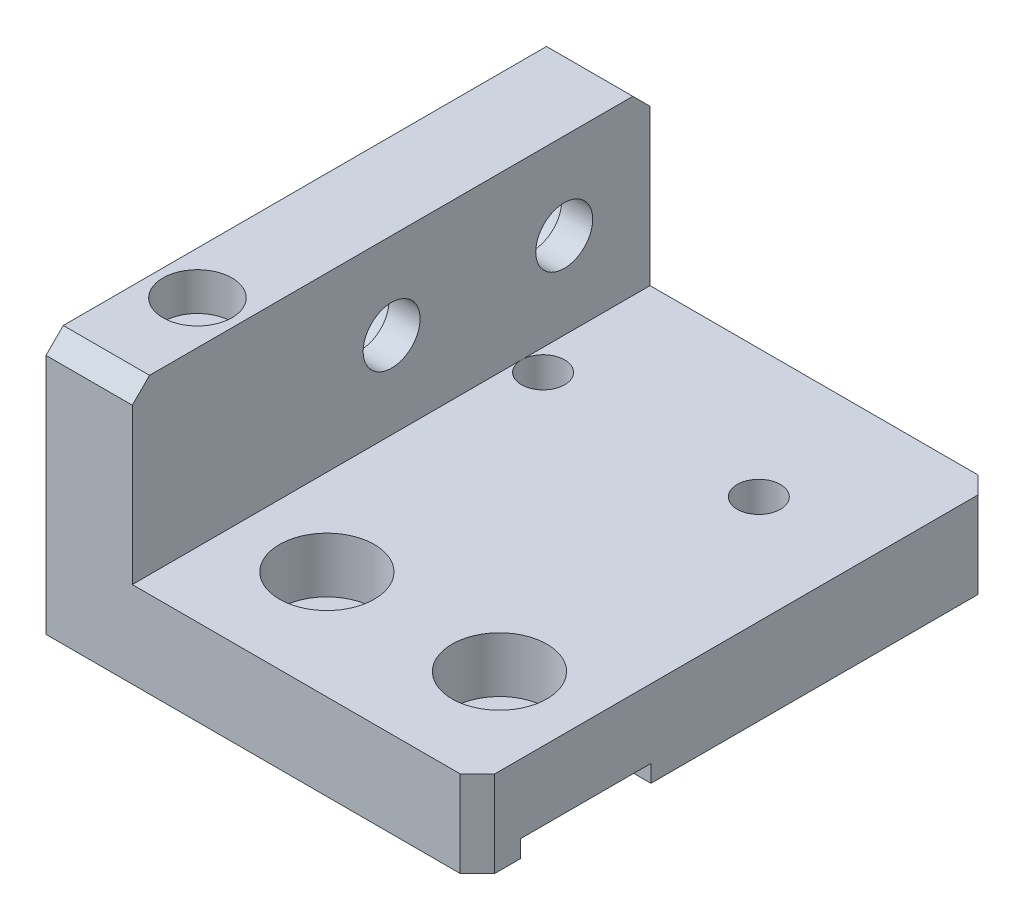
from build123d import *

# Parameters (mm, degrees)
EXTRUDE_1_DEPTH              = 60
SKETCH_3_W                   = 50
SKETCH_3_H                   = 15.1
CUT_EXTRUDE_1_DEPTH          = 2
HOLE_WIZARD_M4_1_D           = 4.5
HOLE_WIZARD_M4_1_CBORE_D     = 8
HOLE_WIZARD_M4_1_CBORE_DEPTH = 4.4
HOLE_WIZARD_M6_1_D           = 6.6
HOLE_WIZARD_M6_1_CBORE_D     = 11
HOLE_WIZARD_M6_1_CBORE_DEPTH = 6.4
HOLE_WIZARD_M6_2_D           = 6.6
HOLE_WIZARD_M6_2_CBORE_D     = 11
HOLE_WIZARD_M6_2_CBORE_DEPTH = 6.4
CHAMFER_1_SIZE               = 2
HOLE_WIZARD_M6_1_2_D         = 5
HOLE_WIZARD_M6_1_2_DEPTH     = 17
HOLE_WIZARD_M6_1_2_TIP       = 1.502151548


with BuildPart() as part:
    # 草图2 → 凸台-拉伸1 (new body)
    with BuildSketch(Plane.XY):
        Polygon((50, 0), (0, 0), (0, 30), (10, 30), (10, 10), (50, 10), align=None)
    extrude(amount=EXTRUDE_1_DEPTH)

    # 草图3 → 切除-拉伸1 (cut)
    with BuildSketch(Plane.XZ):
        with Locations((25, 47.45)):
            Rectangle(SKETCH_3_W, SKETCH_3_H)
    extrude(amount=-CUT_EXTRUDE_1_DEPTH, mode=Mode.SUBTRACT)

    # M4 六角凹头螺钉的柱形沉头孔1 (through all)
    with Locations(Plane(origin=(-8.97546782, 30, 41.476708605), x_dir=(1, 0, 0), z_dir=(0, 1, 0))):
        with Locations((13.97546782, -5.973291395)):
            CounterBoreHole(HOLE_WIZARD_M4_1_D / 2, HOLE_WIZARD_M4_1_CBORE_D / 2, HOLE_WIZARD_M4_1_CBORE_DEPTH)

    # Hole Wizard M6 _1 (through all)
    with Locations(Plane(origin=(0, 10, 0), x_dir=(1, 0, 0), z_dir=(0, 1, 0))):
        with Locations((20, -47.45), (40, -47.45)):
            CounterBoreHole(HOLE_WIZARD_M6_1_D / 2, HOLE_WIZARD_M6_1_CBORE_D / 2, HOLE_WIZARD_M6_1_CBORE_DEPTH)

    # M6 六角凹头螺钉的柱形沉头孔2 (through all)
    with Locations(Plane.ZY):
        with Locations((9.95, 20), (29.95, 20)):
            CounterBoreHole(HOLE_WIZARD_M6_2_D / 2, HOLE_WIZARD_M6_2_CBORE_D / 2, HOLE_WIZARD_M6_2_CBORE_DEPTH)

    # 倒角1
    chamfer_1_edges = [part.edges().sort_by_distance(p)[0] for p in [
        (5, 30, 60),
        (50, 5, 60),
        (5, 30, 0),
        (50, 5, 0),
    ]]
    chamfer(chamfer_1_edges, length=CHAMFER_1_SIZE)

    # Hole Wizard M6 _1 2
    with Locations(Plane(origin=(0, 0, 0), x_dir=(-1, 0, 0), z_dir=(0, -1, 0))):
        with Locations((-12.5, -14.9), (-37.5, -14.9)):
            Hole(HOLE_WIZARD_M6_1_2_D / 2, depth=HOLE_WIZARD_M6_1_2_DEPTH)
            with Locations((0, 0, -(HOLE_WIZARD_M6_1_2_DEPTH + HOLE_WIZARD_M6_1_2_TIP / 2))):  # 118° drill point
                Cone(0, HOLE_WIZARD_M6_1_2_D / 2, HOLE_WIZARD_M6_1_2_TIP, mode=Mode.SUBTRACT)


solid = part.part
